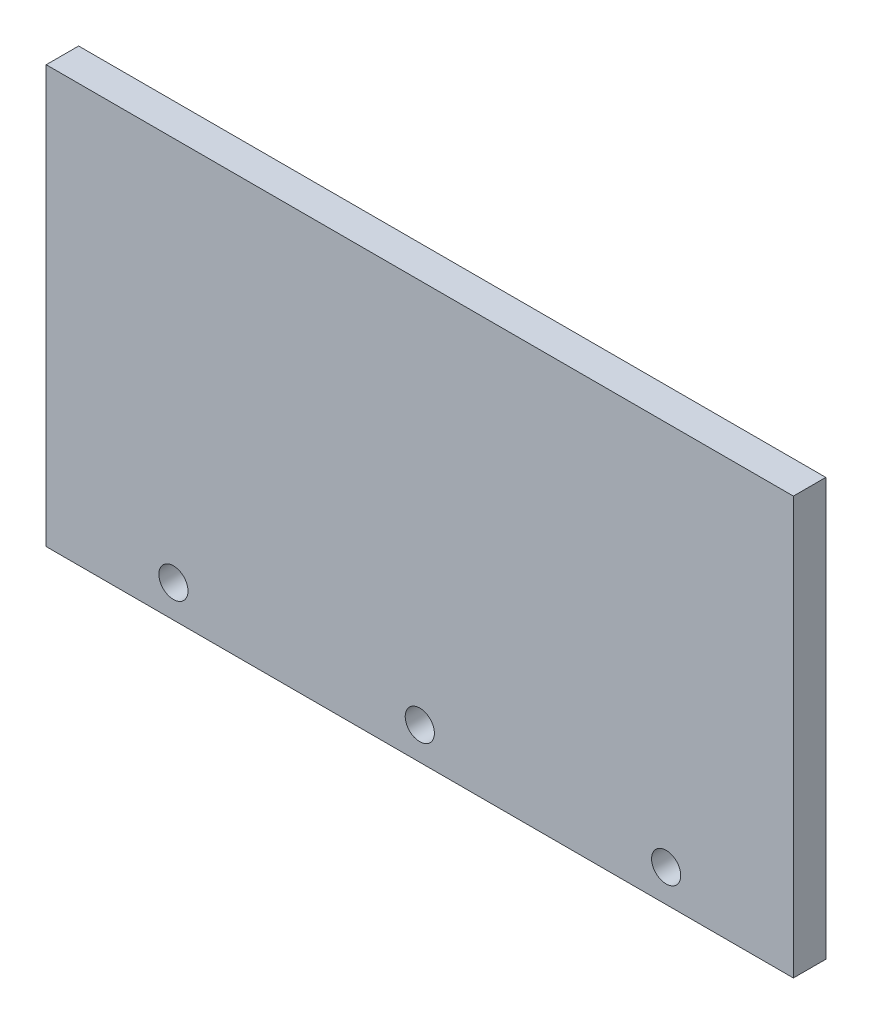
from build123d import *

# Parameters (mm, degrees)
SKETCH1_W           = 922
SKETCH1_H           = 515
SKETCH1_R           = 18
BOSS_EXTRUDE1_DEPTH = 40


with BuildPart() as part:
    # Sketch1 → Boss-Extrude1 (new body)
    with BuildSketch(Plane.XY):
        with Locations((461, 257.5)):
            Rectangle(SKETCH1_W, SKETCH1_H)
        with Locations((461, 40)):
            Circle(SKETCH1_R, mode=Mode.SUBTRACT)
        with Locations((765, 40)):
            Circle(SKETCH1_R, mode=Mode.SUBTRACT)
        with Locations((157, 40)):
            Circle(SKETCH1_R, mode=Mode.SUBTRACT)
    extrude(amount=BOSS_EXTRUDE1_DEPTH)


solid = part.part
